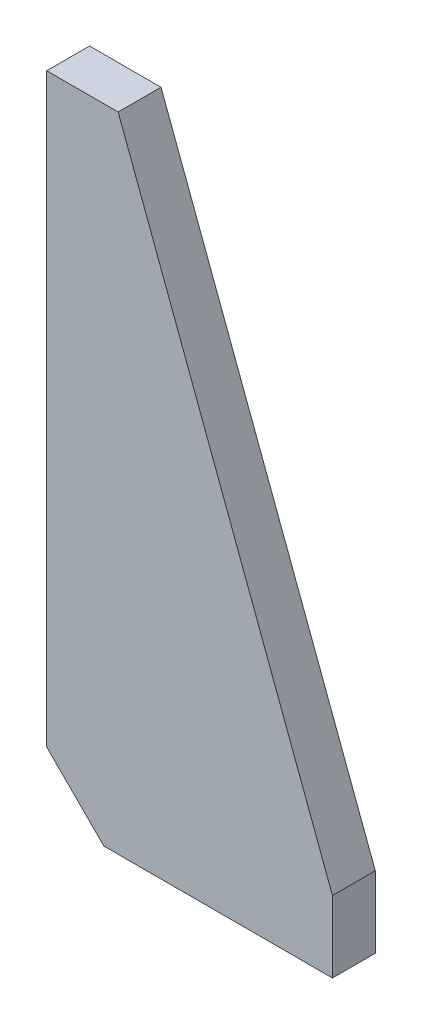
from build123d import *

# Parameters (mm, degrees)
BOSS_EXTRUDE1_DEPTH = 3
CHAMFER1_SIZE       = 8


with BuildPart() as part:
    # Sketch1 → Boss-Extrude1 (new, symmetric)
    with BuildSketch(Plane.XY):
        Polygon((0, 90), (0, 0), (40, 0), (40, 10), (10, 90), align=None)
    extrude(amount=BOSS_EXTRUDE1_DEPTH, both=True)

    # Chamfer1
    chamfer1_edges = [part.edges().sort_by_distance(p)[0] for p in [
        (0, 0, 0),
    ]]
    chamfer(chamfer1_edges, length=CHAMFER1_SIZE)


solid = part.part
